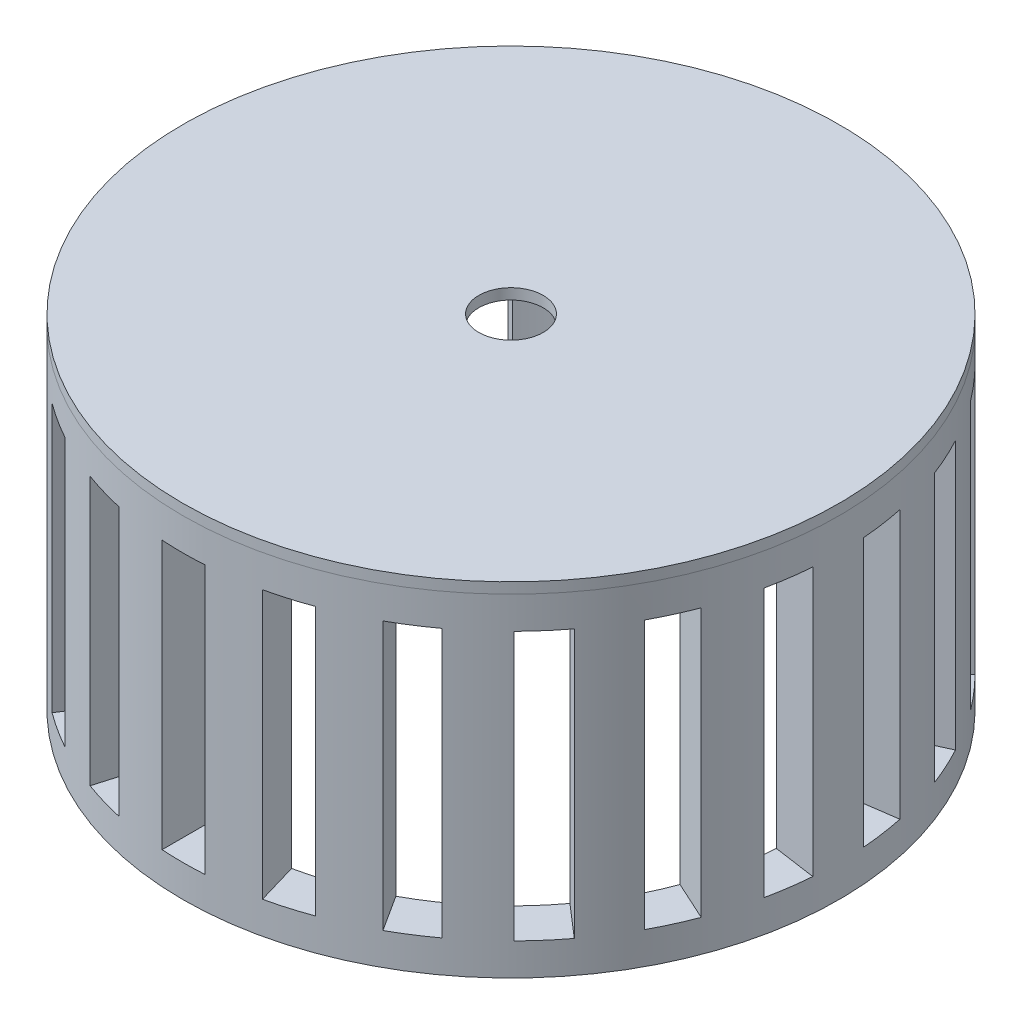
SolidWorks part; units mm, degrees
material "Q235"
ref_plane "Front Plane" through (0, 0, 0) normal (0, 0, 1) x (1, 0, 0)
ref_plane "Top Plane" through (0, 0, 0) normal (0, 1, 0) x (1, 0, 0)
ref_plane "Right Plane" through (0, 0, 0) normal (1, 0, 0) x (0, 0, -1)
sketch "Sketch1" plane through (0, 0, 0) normal (0, 1, 0) x (1, 0, 0)
  circle A0 centre (0, 0) radius 153
  circle A1 centre (0, 0) radius 133
  dimension "D1" = 306
  dimension "D2" = 20
extrude "Boss-Extrude1" add sketch "Sketch1" along normal blind 155
sketch "Sketch2" plane through (0, 0, 0) normal (0, 0, 1) x (1, 0, 0)
  line L0 (0, 0) -> (0, 15) construction
  line L1 (-10, 140) -> (10, 140)
  line L2 (-10, 140) -> (-10, 15)
  line L3 (-10, 15) -> (10, 15)
  line L4 (10, 140) -> (10, 15)
  line L5 (-153, 0) -> (153, 0) construction
  line L6 (153, 155) -> (-153, 155) construction
  dimension "D1" = 15
  dimension "D2" = 15
  dimension "D3" = 20
extrude "Cut-Extrude1" cut sketch "Sketch2" against normal through all both and the other way through all
pattern_circular "CirPattern1" count 22 over 360 about axis through (0, 0, 0) along (0, 1, 0) of "Cut-Extrude1"
sketch "Sketch3" plane through (0, 155, 0) normal (0, 1, 0) x (1, 0, 0)
  circle A1 centre (0, 0) radius 153
  circle A2 centre (0, 0) radius 153
  dimension "D1" = 0
extrude "Boss-Extrude2" add sketch "Sketch3" along normal blind 5 separate body
sketch "Sketch4" plane through (0, 160, 0) normal (0, 1, 0) x (1, 0, 0)
  circle A0 centre (0, 0) radius 15
  dimension "D1" = 30
extrude "Cut-Extrude2" cut sketch "Sketch4" against normal through all
